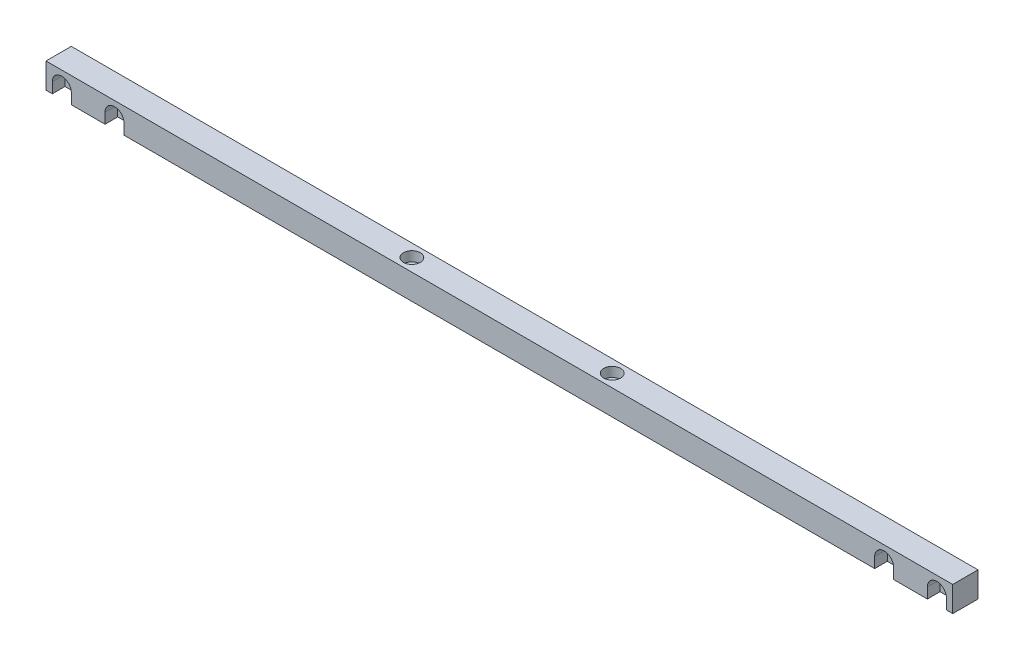
SolidWorks part; units mm, degrees
material "6061 合金"
ref_plane "前视基准面" through (0, 0, 0) normal (0, 0, 1) x (1, 0, 0)
ref_plane "上视基准面" through (0, 0, 0) normal (0, 1, 0) x (1, 0, 0)
ref_plane "右视基准面" through (0, 0, 0) normal (1, 0, 0) x (0, 0, -1)
sketch "草图1" plane through (0, 0, 0) normal (0, 0, 1) x (1, 0, 0)
  line L1 (-215, 6) -> (215, 6)
  line L2 (-215, 6) -> (-215, -6)
  line L3 (-215, -6) -> (215, -6)
  line L4 (215, 6) -> (215, -6)
  line L5 (-215, 6) -> (215, -6) construction
  line L6 (-215, -6) -> (215, 6) construction
  point P0 (0, 0)
  dimension "D1" = 430
  dimension "D2" = 12
extrude "凸台-拉伸1" add sketch "草图1" along normal mid plane 12
hole_wizard "Ø5.5 (5.5) 直径孔1" positions "草图5" profile "草图4" hole size "Ø5.5" standard "GB" end condition through all
sketch "草图5" plane through (0, 0, 6) normal (0, 0, 1) x (1, 0, 0)
  line L0 (-215, 6) -> (-215, -6) construction
  line L1 (215, -6) -> (215, 6) construction
  line L2 (-215, -6) -> (215, -6) construction
  point P0 (-207.5, -1)
  point P2 (-182.5, -1)
  point P4 (182.5, -1)
  point P6 (207.5, -1)
  dimension "D1" = 25
  dimension "D2" = 7.5
  dimension "D3" = 25
  dimension "D4" = 7.5
  dimension "D5" = 5
sketch "草图4" plane through (-207.5, -1, 6) normal (1, 0, 0) x (0, -1, 0)
  line L0 (0, 0) -> (0, 12)
  line L1 (0, 12) -> (2.75, 12)
  line L2 (2.75, 12) -> (2.75, 0)
  line L5 (2.75, 0) -> (0, 0)
  line L11 (0, -6.35) -> (0, 107.95) construction
  dimension "通孔孔直径" = 5.5
  dimension "通孔孔深度" = 12
hole_wizard "打孔尺寸(%根据)内六角圆柱头螺钉的类型2" positions "草图8" profile "草图7" counterbore size "M4" standard "GB"
sketch "草图8" plane through (0, 6, 0) normal (0, 1, 0) x (1, 0, 0)
  point P0 (-47.5, 0)
  point P2 (47.5, 0)
  dimension "D1" = 95
  dimension "D2" = 47.5
sketch "草图7" plane through (-47.5, 6, 0) normal (1, 0, 0) x (0, 0, 1)
  line L0 (0, 0) -> (0, 15.3519)
  line L1 (0, 15.3519) -> (2.25, 14)
  line L2 (2.25, 14) -> (2.25, 4.6)
  line L3 (2.25, 4.6) -> (4, 4.6)
  line L4 (4, 4.6) -> (4, 0)
  line L5 (4, 0) -> (0, 0)
  line L10 (0, 15.3519) -> (-2.25, 14) construction
  line L11 (0, -6.35) -> (0, 107.95) construction
  dimension "孔直径" = 4.5
  dimension "孔深度" = 14
  dimension "柱形沉头孔直径" = 8
  dimension "柱形沉头孔深度" = 4.6
  dimension "导头角度" = 118
sketch "草图9" plane through (0, 0, 6) normal (0, 0, 1) x (1, 0, 0)
  line L0 (-207.5, -1) -> (-207.5, -15.2346) construction
  line L1 (-203, -1) -> (-203, -15.2346)
  line L2 (-212, -1) -> (-212, -15.2346)
  line L3 (-182.5, -1) -> (-182.5, -15.2346) construction
  line L4 (-178, -1) -> (-178, -15.2346)
  line L5 (-187, -1) -> (-187, -15.2346)
  line L6 (182.5, -1) -> (182.5, -15.2346) construction
  line L7 (187, -1) -> (187, -15.2346)
  line L8 (178, -1) -> (178, -15.2346)
  line L9 (207.5, -1) -> (207.5, -15.2346) construction
  line L10 (212, -1) -> (212, -15.2346)
  line L11 (203, -1) -> (203, -15.2346)
  arc A0 (-203, -1) -> (-212, -1) centre (-207.5, -1) ccw
  arc A1 (-212, -15.2346) -> (-203, -15.2346) centre (-207.5, -15.2346) ccw
  arc A2 (-178, -1) -> (-187, -1) centre (-182.5, -1) ccw
  arc A3 (-187, -15.2346) -> (-178, -15.2346) centre (-182.5, -15.2346) ccw
  arc A4 (187, -1) -> (178, -1) centre (182.5, -1) ccw
  arc A5 (178, -15.2346) -> (187, -15.2346) centre (182.5, -15.2346) ccw
  arc A6 (212, -1) -> (203, -1) centre (207.5, -1) ccw
  arc A7 (203, -15.2346) -> (212, -15.2346) centre (207.5, -15.2346) ccw
  point P3 (-207.5, -8.1173)
  point P8 (-182.5, -8.1173)
  point P16 (182.5, -8.1173)
  point P24 (207.5, -8.1173)
  dimension "D1" = 4.5
extrude "切除-拉伸1" cut sketch "草图9" against normal blind 6
